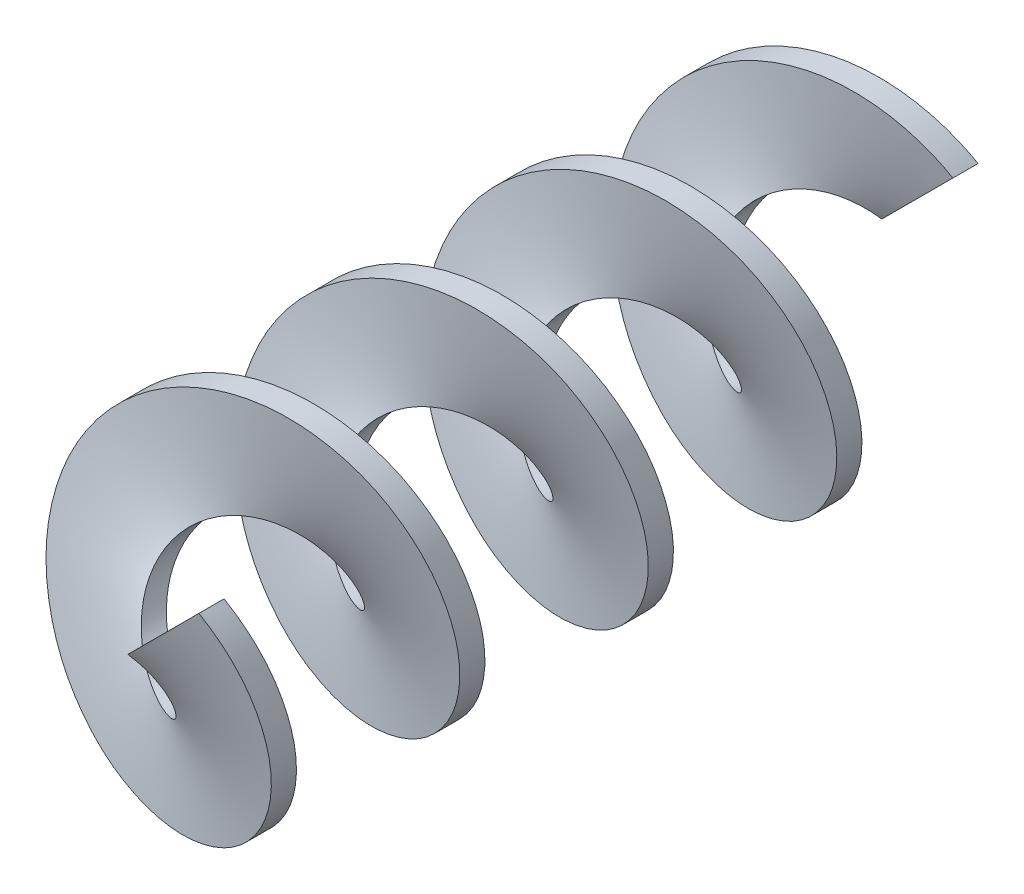
from build123d import *

# Parameters (mm, degrees)
SWEEP1_PITCH       = 3.75
SWEEP1_HEIGHT      = 15
SWEEP1_RADIUS      = 3
SWEEP1_START_ANGLE = 135
SKETCH16_W         = 2
SKETCH16_H         = 0.5


with BuildPart() as part:
    # Sweep1: sweep along a helix
    with BuildLine() as sweep1_path:
        add(Helix(SWEEP1_PITCH, SWEEP1_HEIGHT, SWEEP1_RADIUS, center=(0, 0, 15), direction=(0, 0, -1), mode=Mode.PRIVATE).rotate(Axis((0, 0, 15), (0, 0, -1)), SWEEP1_START_ANGLE))
    # Sketch16 → Sweep1 (sweep)
    with BuildSketch(Plane(origin=(0, 0, 0), x_dir=(1, 0, 0), z_dir=(0, 1, 0))):
        with Locations((2.121320344, -15)):
            Rectangle(SKETCH16_W, SKETCH16_H)
    sweep(path=sweep1_path.line, is_frenet=True)


solid = part.part
